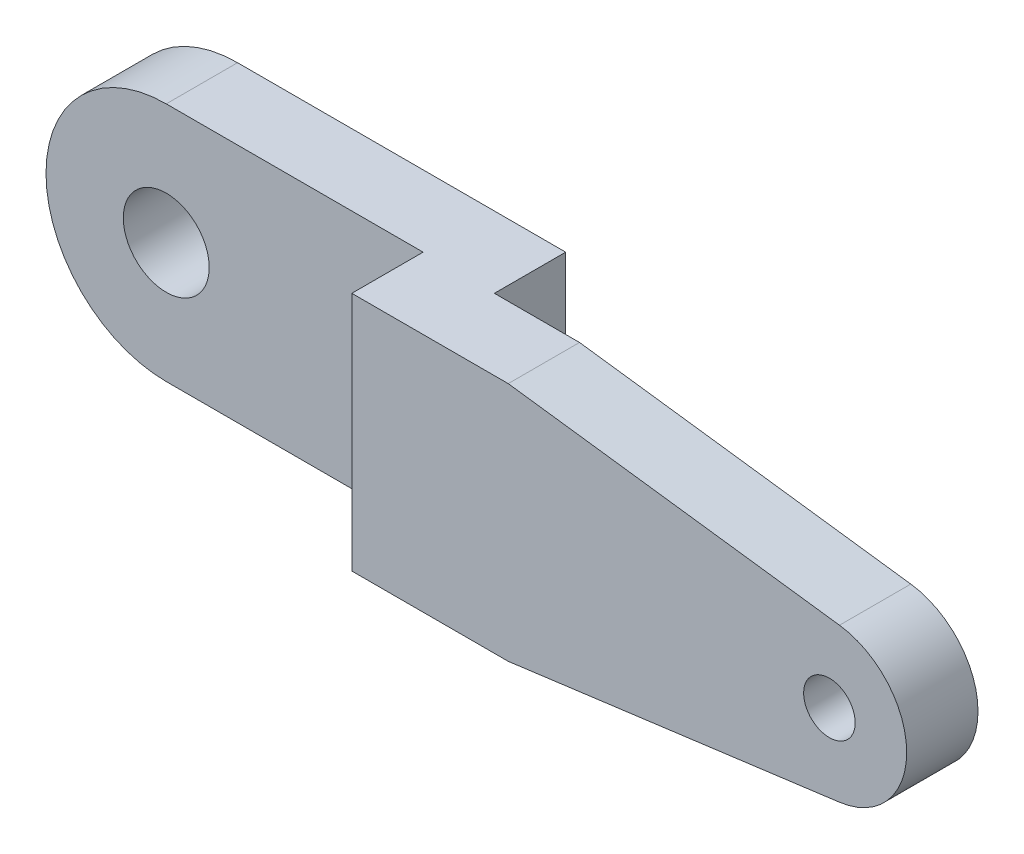
from build123d import *

# Parameters (mm, degrees)
SKETCH1_R           = 5
SKETCH1_W           = 8.3
SKETCH1_H           = 28
BOSS_EXTRUDE2_DEPTH = 8.3
SKETCH2_R           = 3
BOSS_EXTRUDE4_DEPTH = 8.3


with BuildPart() as part:
    # Sketch1 → Boss-Extrude2 (new body)
    # profile 1 of 2: a face of its own
    with BuildSketch(Plane.XY):
        with BuildLine():
            Line((-29.9, 14), (0, 14))
            Line((0, 14), (0, -14))
            Line((0, -14), (-29.9, -14))
            ThreePointArc((-29.9, -14), (-43.9, 0), (-29.9, 14))
        make_face()
        with Locations(Location((-29.9, 0, 0), (0, 0, 180))):
            Circle(SKETCH1_R, mode=Mode.SUBTRACT)
    # profile 2 of 2: a face of its own
    with BuildSketch(Plane.XY):
        with Locations((4.15, 0)):
            Rectangle(SKETCH1_W, SKETCH1_H)
    extrude(amount=BOSS_EXTRUDE2_DEPTH)

    # Sketch2 → Boss-Extrude4 (add)
    with BuildSketch(Plane.XY.offset(8.3)):
        with BuildLine():
            Line((0, 14), (0, -14))
            Line((0, -14), (18.211120602, -14))
            Line((18.211120602, -14), (56.77473573, -8.923003752))
            ThreePointArc((56.77473573, -8.923003752), (64.6, 0), (56.77473573, 8.923003752))
            Line((56.77473573, 8.923003752), (18.211120602, 14))
            Line((18.211120602, 14), (0, 14))
        make_face()
        with Locations(Location((55.6, 0, 0), (0, 0, 180))):
            Circle(SKETCH2_R, mode=Mode.SUBTRACT)
    extrude(amount=BOSS_EXTRUDE4_DEPTH)


solid = part.part
